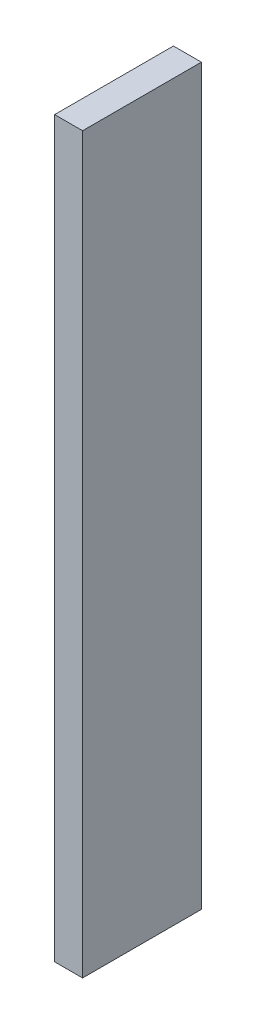
SolidWorks part; units mm, degrees
ref_plane "前视基准面" through (0, 0, 0) normal (0, 0, 1) x (1, 0, 0)
ref_plane "上视基准面" through (0, 0, 0) normal (0, 1, 0) x (1, 0, 0)
ref_plane "右视基准面" through (0, 0, 0) normal (1, 0, 0) x (0, 0, -1)
sketch "草图1" plane through (0, 0, 0) normal (0, 0, 1) x (1, 0, 0)
  line L1 (-4, -105) -> (4, -105)
  line L2 (-4, -105) -> (-4, 105)
  line L3 (-4, 105) -> (4, 105)
  line L4 (4, -105) -> (4, 105)
  line L5 (-4, -105) -> (4, 105) construction
  line L6 (-4, 105) -> (4, -105) construction
  point P0 (0, 0)
  dimension "D1" = 210
  dimension "D2" = 8
extrude "凸台-拉伸1" add sketch "草图1" along normal blind 34
